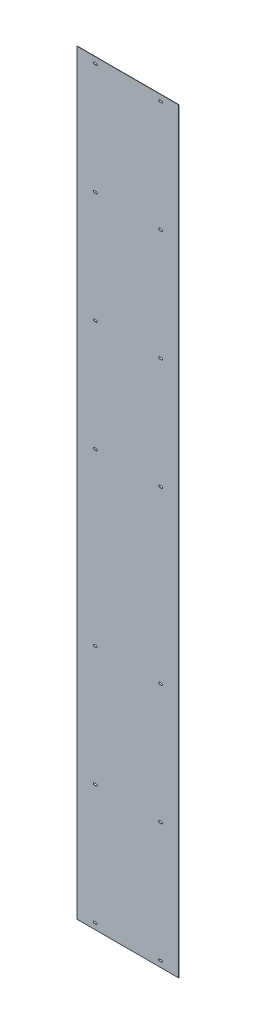
SolidWorks part; units mm, degrees
material "Q235A"
ref_plane "前视基准面" through (0, 0, 0) normal (0, 0, 1) x (1, 0, 0)
ref_plane "上视基准面" through (0, 0, 0) normal (0, 1, 0) x (1, 0, 0)
ref_plane "右视基准面" through (0, 0, 0) normal (1, 0, 0) x (0, 0, -1)
sketch "草图1" plane through (0, 0, 0) normal (0, 0, 1) x (1, 0, 0)
  line L1 (-161, 1197) -> (161, 1197)
  line L2 (-161, 1197) -> (-161, -1197)
  line L3 (-161, -1197) -> (161, -1197)
  line L4 (161, 1197) -> (161, -1197)
  line L5 (-161, 1197) -> (161, -1197) construction
  line L6 (-161, -1197) -> (161, 1197) construction
  point P0 (0, 0)
extrude "凸台-拉伸1" add sketch "草图1" along normal blind 0.8
sketch "草图2" plane through (0, 0, 0.8) normal (0, 0, 1) x (1, 0, 0)
  line L0 (-103.5, 1197) -> (-103.5, -1197) construction
  line L1 (161, 1197) -> (-161, 1197) construction
  line L2 (-161, -1197) -> (161, -1197) construction
  line L3 (0, 1197) -> (0, -1197) construction
  line L4 (-161, 1197) -> (-161, -1197) construction
  line L5 (-106.5, 121) -> (-100.5, 121) construction
  line L6 (-106.5, 1178) -> (-100.5, 1178) construction
  line L7 (-106.5, 124) -> (-100.5, 124)
  line L8 (-106.5, 118) -> (-100.5, 118)
  line L9 (-106.5, 1181) -> (-100.5, 1181)
  line L10 (-106.5, 1175) -> (-100.5, 1175)
  line L11 (-106.5, -1178) -> (-100.5, -1178) construction
  line L14 (-106.5, 825.6667) -> (-100.5, 825.6667) construction
  line L15 (-106.5, 828.6667) -> (-100.5, 828.6667)
  line L16 (-106.5, 822.6667) -> (-100.5, 822.6667)
  line L17 (-106.5, -1175) -> (-100.5, -1175)
  line L20 (-106.5, 473.3333) -> (-100.5, 473.3333) construction
  line L21 (-106.5, 476.3333) -> (-100.5, 476.3333)
  line L22 (-106.5, 470.3333) -> (-100.5, 470.3333)
  line L23 (-106.5, -1181) -> (-100.5, -1181)
  line L26 (106.5, -1178) -> (100.5, -1178) construction
  line L29 (-106.5, -798.5) -> (-100.5, -798.5) construction
  line L32 (-106.5, -795.5) -> (-100.5, -795.5)
  line L33 (-106.5, -801.5) -> (-100.5, -801.5)
  line L34 (-106.5, -419) -> (-100.5, -419) construction
  line L35 (-106.5, -416) -> (-100.5, -416)
  line L36 (-106.5, -422) -> (-100.5, -422)
  line L37 (106.5, -1175) -> (100.5, -1175)
  line L38 (106.5, -1181) -> (100.5, -1181)
  line L39 (106.5, -798.5) -> (100.5, -798.5) construction
  line L40 (106.5, -795.5) -> (100.5, -795.5)
  line L41 (106.5, -801.5) -> (100.5, -801.5)
  line L42 (106.5, -419) -> (100.5, -419) construction
  line L43 (106.5, -416) -> (100.5, -416)
  line L44 (106.5, -422) -> (100.5, -422)
  line L45 (106.5, 473.3333) -> (100.5, 473.3333) construction
  line L46 (106.5, 476.3333) -> (100.5, 476.3333)
  line L47 (106.5, 470.3333) -> (100.5, 470.3333)
  line L48 (106.5, 825.6667) -> (100.5, 825.6667) construction
  line L49 (106.5, 828.6667) -> (100.5, 828.6667)
  line L50 (106.5, 822.6667) -> (100.5, 822.6667)
  line L51 (106.5, 1178) -> (100.5, 1178) construction
  line L52 (106.5, 1181) -> (100.5, 1181)
  line L53 (106.5, 1175) -> (100.5, 1175)
  line L54 (106.5, 121) -> (100.5, 121) construction
  line L55 (106.5, 124) -> (100.5, 124)
  line L56 (106.5, 118) -> (100.5, 118)
  line L57 (161, 100) -> (-161, 100) construction
  line L58 (161, 100) -> (161, -400) construction
  line L59 (161, -400) -> (-161, -400) construction
  line L60 (-161, 100) -> (-161, -400) construction
  line L61 (161, 100) -> (-161, -400) construction
  line L62 (161, -400) -> (-161, 100) construction
  line L63 (-103.5, -1178) -> (-83.5, -1178) construction
  line L64 (-83.5, -1178) -> (-83.5, -419) construction
  line L65 (-83.5, -419) -> (-103.5, -419) construction
  line L66 (-83.5, -798.5) -> (-103.5, -798.5) construction
  line L67 (-103.5, 121) -> (-83.5, 121) construction
  line L68 (-83.5, 121) -> (-83.5, 473.3333) construction
  line L69 (-83.5, 473.3333) -> (-83.5, 825.6667) construction
  line L70 (-83.5, 825.6667) -> (-83.5, 1178) construction
  line L71 (-83.5, 1178) -> (-103.5, 1178) construction
  line L72 (-83.5, 825.6667) -> (-103.5, 825.6667) construction
  line L73 (-83.5, 473.3333) -> (-103.5, 473.3333) construction
  arc A26 (-106.5, 1181) -> (-106.5, 1175) centre (-106.5, 1178) ccw
  arc A27 (-100.5, 1175) -> (-100.5, 1181) centre (-100.5, 1178) ccw
  arc A30 (-106.5, 828.6667) -> (-106.5, 822.6667) centre (-106.5, 825.6667) ccw
  arc A31 (-100.5, 822.6667) -> (-100.5, 828.6667) centre (-100.5, 825.6667) ccw
  arc A34 (-106.5, 476.3333) -> (-106.5, 470.3333) centre (-106.5, 473.3333) ccw
  arc A35 (-100.5, 470.3333) -> (-100.5, 476.3333) centre (-100.5, 473.3333) ccw
  arc A42 (-106.5, -1175) -> (-106.5, -1181) centre (-106.5, -1178) ccw
  arc A43 (-100.5, -1181) -> (-100.5, -1175) centre (-100.5, -1178) ccw
  arc A44 (-106.5, -795.5) -> (-106.5, -801.5) centre (-106.5, -798.5) ccw
  arc A45 (-100.5, -801.5) -> (-100.5, -795.5) centre (-100.5, -798.5) ccw
  arc A46 (-106.5, -416) -> (-106.5, -422) centre (-106.5, -419) ccw
  arc A47 (-100.5, -422) -> (-100.5, -416) centre (-100.5, -419) ccw
  arc A48 (106.5, -1175) -> (106.5, -1181) centre (106.5, -1178) cw
  arc A49 (100.5, -1181) -> (100.5, -1175) centre (100.5, -1178) cw
  arc A50 (106.5, -795.5) -> (106.5, -801.5) centre (106.5, -798.5) cw
  arc A51 (100.5, -801.5) -> (100.5, -795.5) centre (100.5, -798.5) cw
  arc A52 (106.5, -416) -> (106.5, -422) centre (106.5, -419) cw
  arc A53 (100.5, -422) -> (100.5, -416) centre (100.5, -419) cw
  arc A54 (106.5, 476.3333) -> (106.5, 470.3333) centre (106.5, 473.3333) cw
  arc A55 (100.5, 470.3333) -> (100.5, 476.3333) centre (100.5, 473.3333) cw
  arc A56 (106.5, 828.6667) -> (106.5, 822.6667) centre (106.5, 825.6667) cw
  arc A57 (100.5, 822.6667) -> (100.5, 828.6667) centre (100.5, 825.6667) cw
  arc A58 (106.5, 1181) -> (106.5, 1175) centre (106.5, 1178) cw
  arc A59 (100.5, 1175) -> (100.5, 1181) centre (100.5, 1178) cw
  arc A60 (-106.5, 124) -> (-106.5, 118) centre (-106.5, 121) ccw
  arc A61 (-100.5, 118) -> (-100.5, 124) centre (-100.5, 121) ccw
  arc A62 (106.5, 124) -> (106.5, 118) centre (106.5, 121) cw
  arc A63 (100.5, 118) -> (100.5, 124) centre (100.5, 121) cw
  point P8 (0, -150)
  point P14 (-103.5, 1178)
  point P19 (-103.5, -1178)
  point P25 (-103.5, -798.5)
  point P27 (-103.5, 825.6667)
  point P39 (-103.5, -419)
  point P42 (-103.5, 473.3333)
  point P54 (-103.5, 121)
  point P57 (103.5, -1178)
  point P64 (103.5, -798.5)
  point P71 (103.5, -419)
  point P78 (103.5, 473.3333)
  point P85 (103.5, 825.6667)
  point P92 (103.5, 1178)
  point P103 (103.5, 121)
  dimension "D3" = 3
  dimension "D4" = 6
  dimension "D5" = 500
  dimension "D6" = 19
  dimension "D7" = 1347
  dimension "D8" = 19
  dimension "D9" = 20
  dimension "D10" = 21
  dimension "D11" = 20
  dimension "D21" = 207
  dimension "D1" = 19
extrude "3001" cut sketch "草图2" against normal blind 10
equation "\"A\" =1195"
equation "\"B\" =1155"
equation "\"CH\" = 2300"
equation "\"OP\" =750"
equation "\"OPH\" = 2100"
equation "\"QB\" = 50"
equation "\"DK\" = 40"
equation "\"WCOP\" =0"
equation "\"HCOP\" =4"
equation "\"FJ\" = 2"
equation "\"DH\" = 16"
equation "\"LG\" = 1"
equation "\"DD\" = 2"
equation "\"C\" =545"
equation "\"PX\" =-75"
equation "\"LZ\" = 350"
equation "\"LJ\" = 1158"
equation "\"LLK\" = 310"
equation "\"FS\" = 0"
equation "\"D2@草图1\"=\"CH\" + \"DH\" + 78"
equation "\"D1@草图1\"=\"LZ\"-28"
equation "\"Bh\"= \"D1@凸台-拉伸1\""
